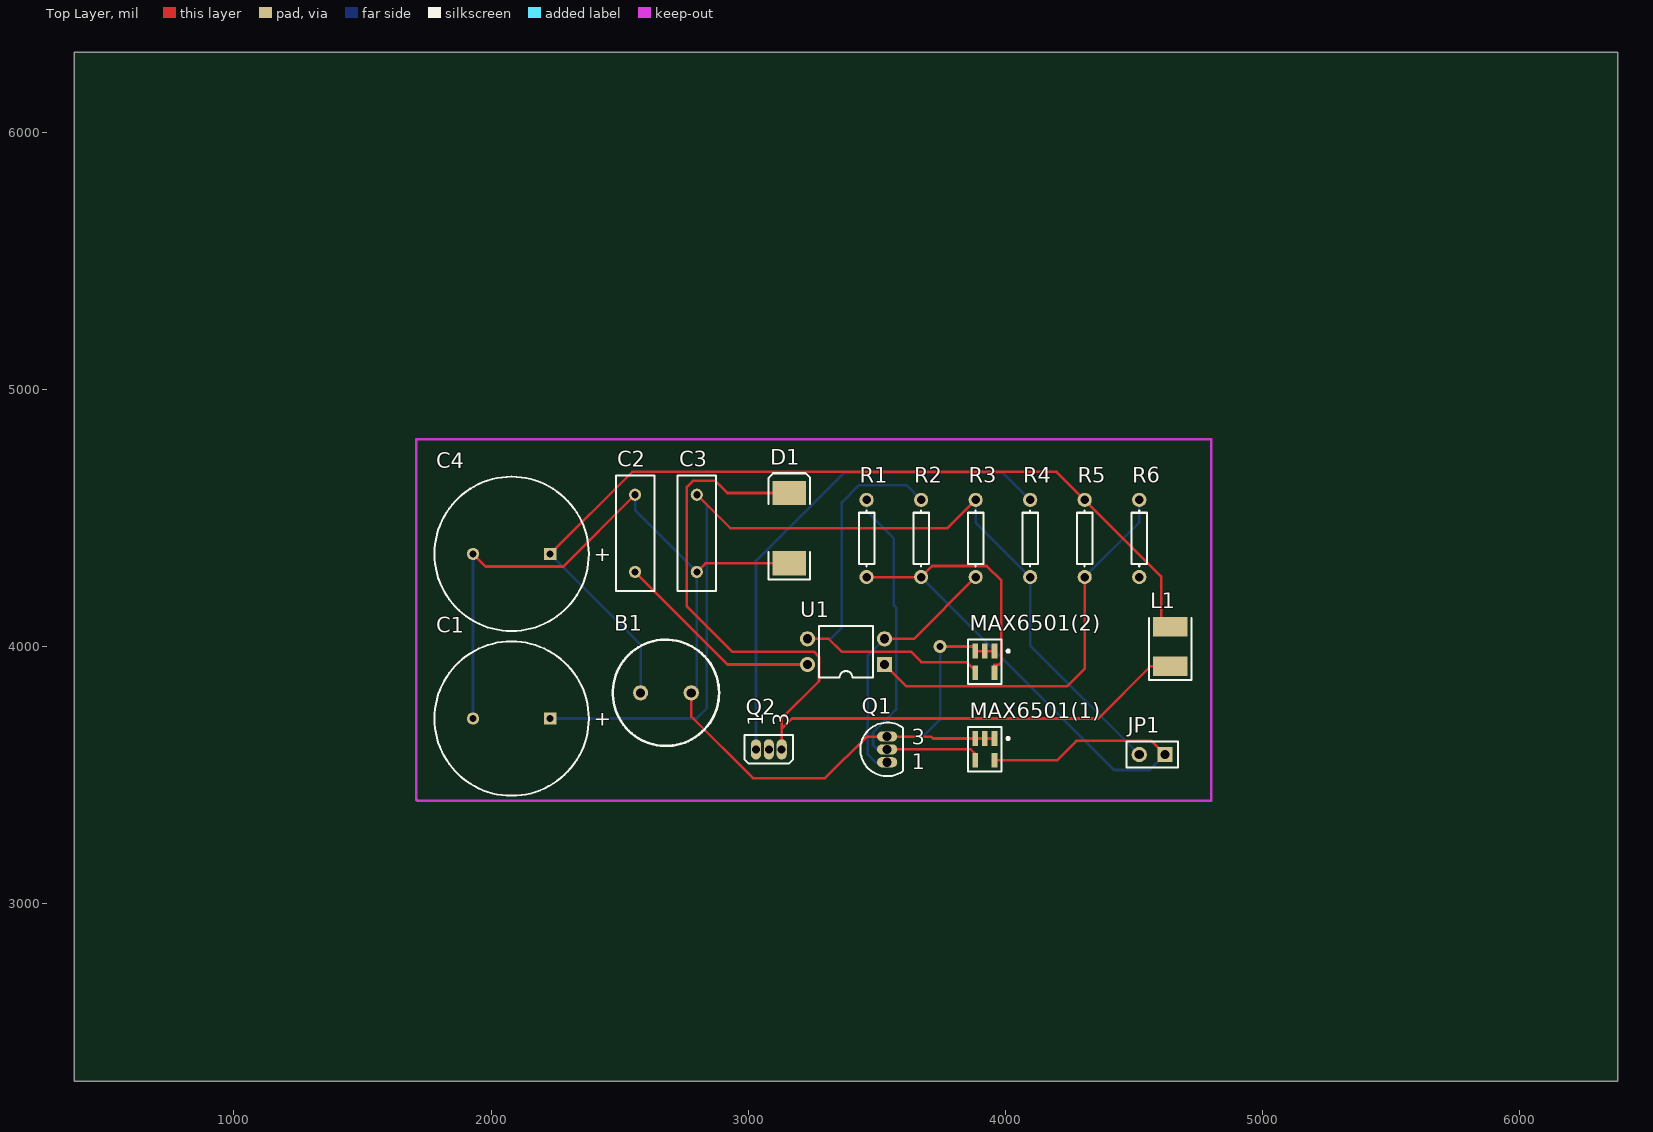
[diagram p0: Top Layer view]
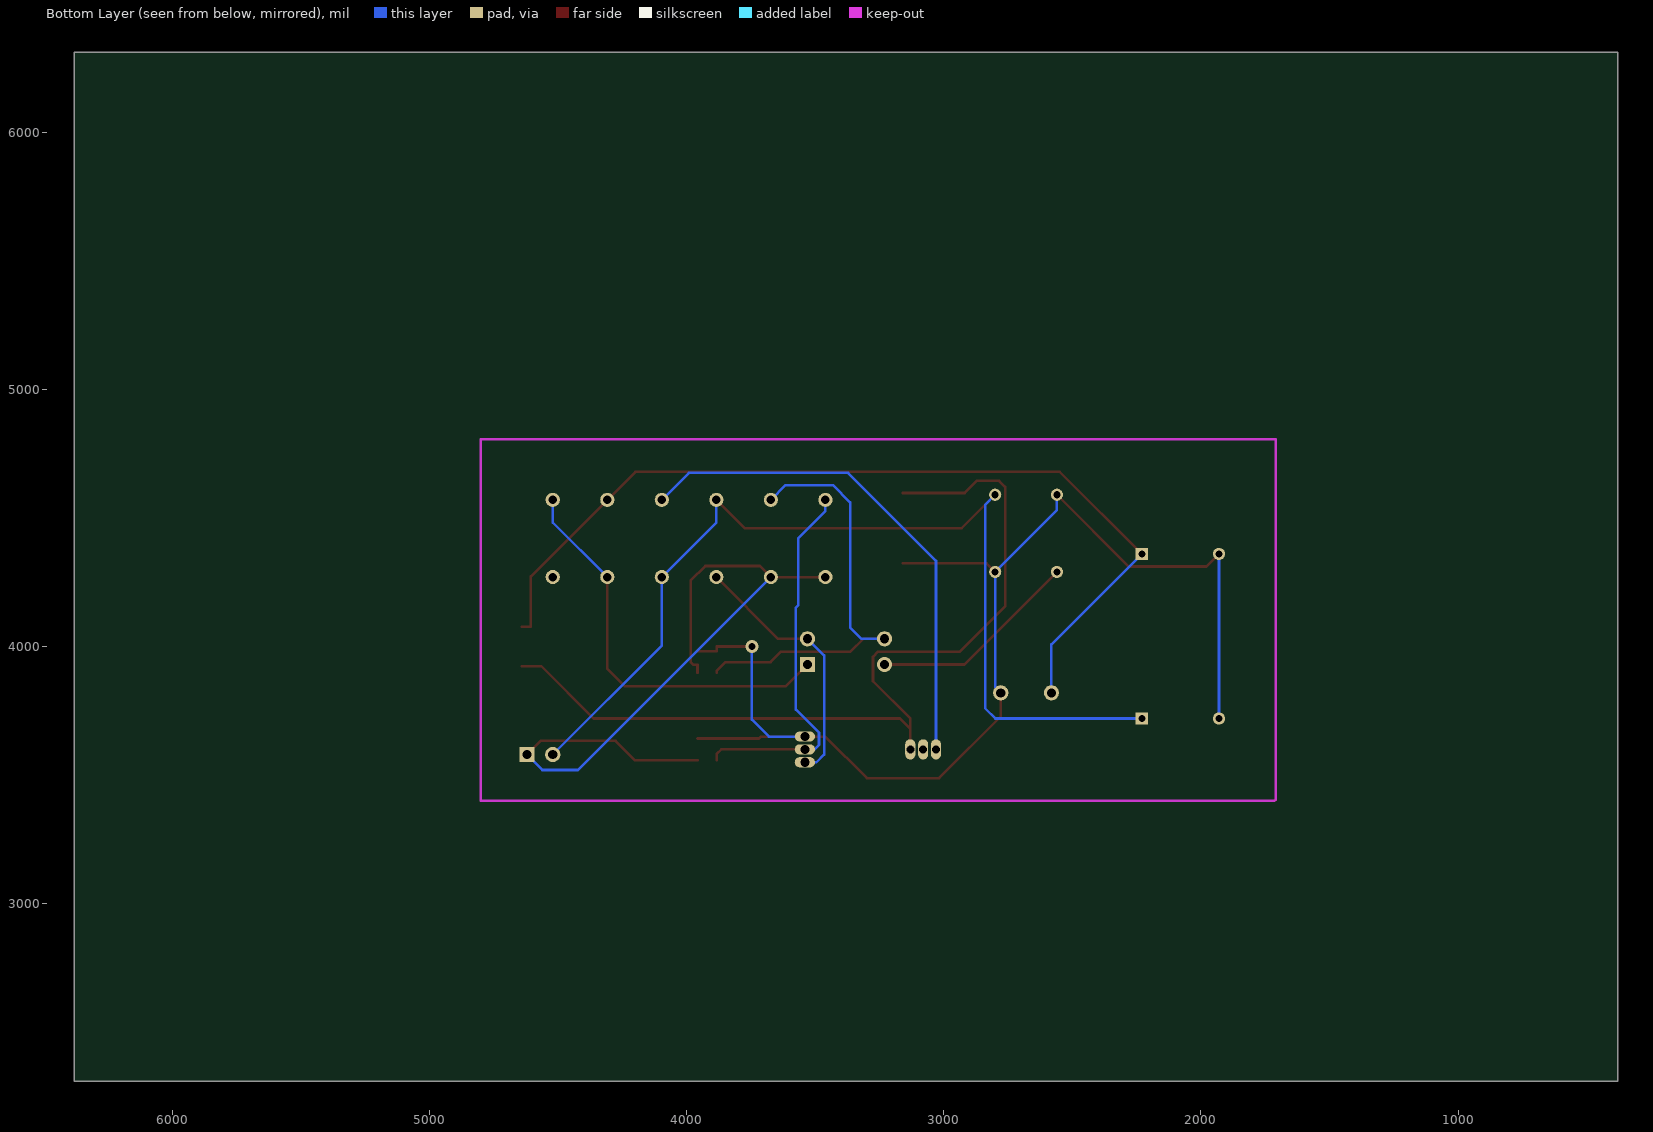
[diagram p1: Bottom Layer view, seen from below]
# Altium PCB MISC95141.PCBDOC
Units mil, origin at the board's own origin, x right, y up, seen from the top; angles counter-clockwise.
Board outline 6000 x 4000 mil, 2 copper layers (Top Layer, Bottom Layer); 19 components, 12 nets, 48 pads, 1 vias.

## Layer stack, top to bottom (the 12.6 mil dielectric is the usual default, probably not edited)
Top Layer: signal copper 1.4
Dielectric: dielectric 12.6, FR-4, Dk 4.8
Bottom Layer: signal copper 1.4

## Board outline
380,2310 6380,2310 6380,6310 380,6310

## Design rules (kind name [scope] priority, off if disabled: settings)
Clearance [All] p1: gap=10
ComponentClearance [All] p1: gap=10 collisioncheckmode=0
PolygonConnect [All] p1: connectstyle=Relief reliefconductorwidth=10 reliefentries=4 polygonreliefangle="90 Angle"
RoutingLayers [All] p1: top layer=Horizontal bottom layer=Vertical
RoutingVias [All] p1: holewidth=28 width=50 viastyle="Through Hole" minholewidth=28 minwidth=50 maxholewidth=28 maxwidth=50
SolderMaskExpansion [All] p1: expansion=4
TestPointUsage [All] p1: valid=0 allowmultiple=FALSE
Testpoint [All] p1: side=15 testpointundercomponent=TRUE minsize=40 maxsize=100 preferedsize=60 minholesize=0 maxholesize=40 preferedholesize=32 testpointgrid=1 style=1023 order=1234567890
Width [All] p1: maxlimit=10 minlimit=10 preferedwidth=10
16 further rules are at their usual default settings.

## Components (designator, comment, footprint, x,y, rotation, side; value= is the part's Value field where it differs from the comment)
B1 "Motor" RB5-10.5 2680,3820 r0 top
C1 "Cap Pol1" RB7.6-15 2080,3720 r0 top
C2 "Cap" RAD-0.3 2560,4440 r270 top
C3 "Cap" RAD-0.3 2800,4440 r90 top
C4 "Cap Pol1" RB7.6-15 2080,4360 r0 top
D1 "Diode" DSO-C2/X3.3 3160,4460 r90 top
JP1 "Header 2" HDR1X2 4620,3580 r180 top
L1 "Inductor" CC4532-1812 4640,4000 r90 top
MAX6501(1) "MAX6501" SO-G5/P.95 3920,3600 r180 top
MAX6501(2) "MAX6501" SO-G5/P.95 3920,3940 r180 top
Q1 "NPN" BCY-W3 3540,3600 r0 top
Q2 "IRF7416" BCY-W3/H.8 3080,3600 r90 top
R1 "Res1" AXIAL-0.3 3460,4420 r90 top
R2 "Res1" AXIAL-0.3 3672,4420 r90 top
R3 "Res1" AXIAL-0.3 3884,4420 r90 top
R4 "Res1" AXIAL-0.3 4096,4420 r90 top
R5 "Res1" AXIAL-0.3 4308,4420 r90 top
R6 "Res1" AXIAL-0.3 4520,4420 r90 top
U1 "MAX1626" DIP-4 3380,3980 r90 top

## Footprints (in the part's own frame and the unit in brackets; to place one, negate y for a bottom-side part, rotate by r counter-clockwise, add the part's x,y. Pads: shape width x height; smd on the part's side, far side on the other; paste and mask are expansions set on the pad)
AXIAL-0.3 [mm]
  round 1.4 hole 0.85: 1(-3.81,0) 2(3.81,0)
  silkscreen extent -2.77,-0.76 2.77,0.76
BCY-W3 [mm]
  oval 2x1 hole 0.9: 1(0,-1.27) 2(0,0) 3(0,1.27)
  silkscreen extent -2.65,-2.65 1.55,2.65
BCY-W3/H.8 [mm]
  oval 2x1 hole 0.8: 1(0,1.27) 2(0,0) 3(0,-1.27)
  silkscreen extent -1.41,-2.41 1.41,2.41
CC4532-1812 [mm]
  rect 1.9x3.4 smd: 1(-1.95,0) 2(1.95,0)
  silkscreen extent -3.3,-2.1 2.8,2.1
DIP-4 [mm]
  rect 1.5x1.5 hole 0.9: 1(-1.27,-3.81)
  round 1.5 hole 0.9: 2(1.27,-3.81) 3(1.27,3.81) 4(-1.27,3.81)
  silkscreen extent -2.55,-2.65 2.55,2.65
DSO-C2/X3.3 [mm]
  rect 2.4x3.3 smd: 1(-3.475,0) 2(3.475,0)
  silkscreen extent -5.08,-2.05 5.42,2.06
HDR1X2 [mm] "Connector; Header; 2 Position"
  rect 1.5x1.5 hole 0.9: 1(0,0)
  round 1.5 hole 0.9: 2(2.54,0)
  silkscreen extent -1.27,-1.27 3.81,1.27
RAD-0.3 [mm]
  round 1.2 hole 0.7: 1(-3.81,0) 2(3.81,0)
  silkscreen extent -5.71,-1.91 5.71,1.91
RB5-10.5 [mm]
  round 1.5 hole 0.9: 1(-2.5,0) 2(2.5,0)
  silkscreen extent -5.25,-5.25 5.25,5.25
RB7.6-15 [mm]
  rect 1.2x1.2 hole 0.7: 1(3.81,0)
  round 1.2 hole 0.7: 2(-3.81,0)
  silkscreen extent -7.62,-7.62 7.62,7.62
SO-G5/P.95 [mm]
  rect 0.55x1.45 smd: 1(-0.95,-1.075) 2(0,-1.075) 3(0.95,-1.075) 4(0.95,1.075) 5(-0.95,1.075)
  silkscreen extent -2.43,-2.2 1.65,2.2

## Part data
B1: "Motor, General Kind"
C1 C4: "Polarized Capacitor (Radial)"
C2 C3: "Capacitor"
D1: "Default Diode"
JP1: "Header, 2-Pin"
Q1: "NPN Bipolar Transistor"
Q2: library part MOSFET-P, "P-Channel MOSFET"
R1 R2 R3 R4 R5 R6: "Resistor"

## Via types
v1: diameter 50, hole 28, Top Layer to Bottom Layer, 1 vias

## Nets (pads, with @x,y where several pads share a name; then routed paths per layer and width w, separated by ;. In a path a pad name is that pad's centre, name@x,y a point inside that pad or via, vN(x,y) a via of type N, cw(c..) or ccw(c..) an arc to the next point about the centre after c; other vN are vias at no path point)
GND: B1.2 C1.2 C2.1 C3.1 C4.2 D1.1 MAX6501(1).1 MAX6501(1).2 MAX6501(1).3 MAX6501(2).1 MAX6501(2).2 MAX6501(2).3 Q1.3 | length 4845
  Top Layer w10: C4.2 1979,4311 2281,4311 C2.1 ; B1.2 2778.43,3728 3018.43,3488 3299,3488 3461,3650 Q1.3 3711,3650 3718.68,3642.32 3882.6,3642.32 3920,3642.32 3957.4,3642.32 ; C3.1 2833.19,4323.19 D1.1 ; v1(3746,4000) 3882.6,4000 3882.6,3982.32 3920,3982.32 3957.4,3982.32
  Bottom Layer w10: C1.2 C4.2 ; C2.1 2560,4530 C3.1 2800,3841.57 B1.2 ; Q1.3 3680,3650 3746,3716 v1(3746,4000)
NetB1_1: B1.1 C4.1 L1.2 R5.2 | length 3592.2
  Top Layer w10: C4.1 2549,4679 4199,4679 R5.2 4605,4273 4605,4076.77 L1.2
  Bottom Layer w10: C4.1 2581.57,4008.43 B1.1
NetC1_1: C1.1 C3.2 JP1.2 R3.2 R4.1 | length 3908.6
  Top Layer w10: C3.2 2930,4460 3774,4460 R3.2
  Bottom Layer w10: C1.1 2799,3720 2839,3760 2839,4551 C3.2 ; R3.2 3884,4482 R4.1 4096,4004 JP1.2
NetC2_2: C2.2 U1.4 | length 819.1
  Top Layer w10: C2.2 2920,3930 U1.4
NetD1_2: D1.2 L1.1 Q2.3 | length 3518.5
  Top Layer w10: Q2.3 3130,3680 ; D1.2 2919.19,4596.81 2872,4644 2785,4644 2761,4620 2761,4156 2937,3980 3255,3980 3275,3960 3275,3865 3130,3720 3130,3680 ; L1.1 4564,3923.23 4360.77,3720 3170,3720 3130,3680
NetJP1_1: JP1.1 MAX6501(1).5 MAX6501(2).5 R1.1 R2.1 | length 2943.2
  Top Layer w10: R1.1 R2.1 3715,4313 3927,4313 3984,4256 3984,3940 3973,3929 3957.4,3929 3957.4,3897.68 ; 3957.4,3557.68 4200.68,3557.68 4276,3633 4567,3633 JP1.1
  Bottom Layer w10: R2.1 4422,3520 4560,3520 JP1.1
NetMAX6501(1)_4: MAX6501(1).4 Q1.2 R1.2 | length 1474
  Top Layer w10: Q1.2 3865,3600 3882.6,3582.4 3882.6,3557.68
  Bottom Layer w10: R1.2 3460,4526 3566,4420 3566,4160 3575,4151 3575,3755 3485,3665 3485,3618 3503,3600 Q1.2
NetMAX6501(2)_4: MAX6501(2).4 R2.2 U1.3 | length 1708.7
  Top Layer w10: U1.3 3313,4030 3363,3980 3632,3980 3673,3939 3847.6,3939 3882.6,3904 3882.6,3897.68
  Bottom Layer w10: U1.3 3320,4030 3364,4074 3364,4560 3431,4627 3615,4627 R2.2
NetQ1_1: Q1.1 R3.1 U1.2 | length 1017.8
  Top Layer w10: U1.2 3644,4030 R3.1
  Bottom Layer w10: U1.2 3465,3965 3465,3580 3495,3550 Q1.1
NetQ2_1: Q2.1 R4.2 | length 1984.2
  Bottom Layer w10: Q2.1 3030,4333 3372,4675 3991,4675 R4.2
NetQ2_2: Q2.2
NetR5_1: R5.1 R6.2 U1.1 | length 1586.2
  Top Layer w10: U1.1 3615,3845 4240,3845 4308,3913 R5.1
  Bottom Layer w10: R5.1 4520,4482 R6.2
pads on no net: R6.1
copper on no net: | length 7.1
  Top Layer w10: 1710,3405 1715,3400

## Keep-outs
Keep-Out Layer:
  lines w10: 1710,3405 1710,4805 4800,4805 ; 1715,3400 4800,3400 4800,4800